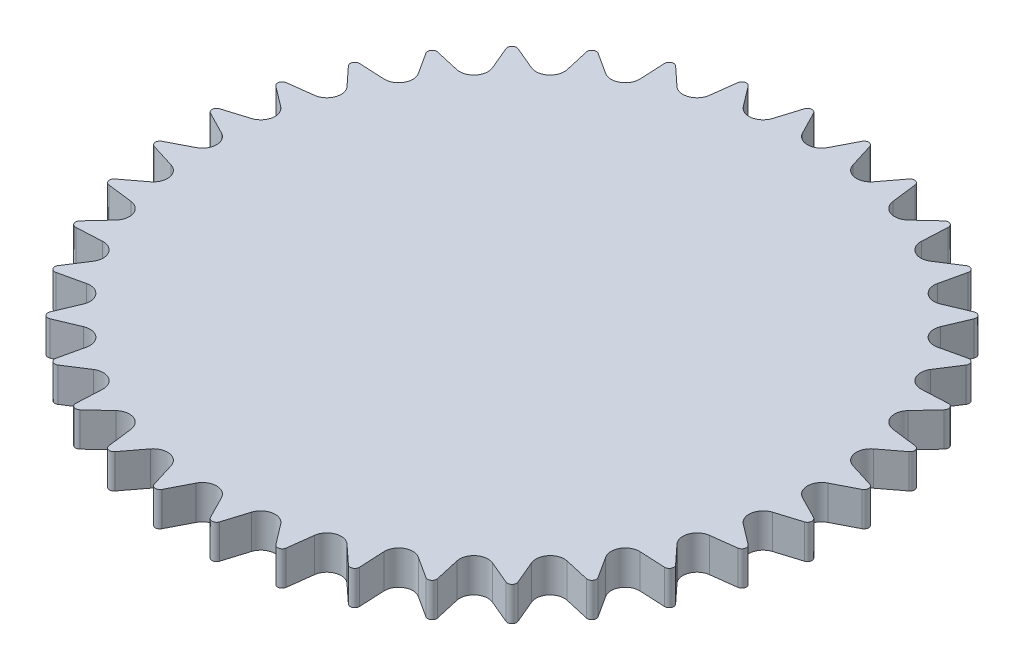
from build123d import *

# Parameters (mm, degrees)
SKETCH_1_R          = 290
BOSS_EXTRUDE1_DEPTH = 30
SKETCH_4_R          = 330.934744746
CUT_EXTRUDE1_DEPTH  = 30


with BuildPart() as part:
    # 草图1 → Boss-Extrude1 (new body)
    with BuildSketch(Plane(origin=(0, 0, 0), x_dir=(1, 0, 0), z_dir=(0, 1, 0))):
        with Locations(Location((0, 0, 0), (0, 0, 270))):
            Circle(SKETCH_1_R)
    extrude(amount=BOSS_EXTRUDE1_DEPTH)

    # 草图4 → Cut-Extrude1 (cut)
    with BuildSketch(Plane(origin=(0, 30, 0), x_dir=(1, 0, 0), z_dir=(0, 1, 0))):
        Circle(SKETCH_4_R)
        with BuildLine():
            Line((-21.368609629, 286.739555153), (-11.118539989, 266.787901567))
            ThreePointArc((-11.118539989, 266.787901567), (0, 260), (11.118539989, 266.787901567))
            Line((11.118539989, 266.787901567), (21.368609629, 286.739555153))
            ThreePointArc((21.368609629, 286.739555153), (22.993156883, 288.413400425), (25.275165397, 288.896462447))
            ThreePointArc((25.275165397, 288.896462447), (27.438622234, 288.024472603), (28.747828783, 286.093957131))
            Line((28.747828783, 286.093957131), (35.377608547, 264.66550808))
            ThreePointArc((35.377608547, 264.66550808), (45.148526193, 256.050015783), (57.276857314, 260.804079666))
            Line((57.276857314, 260.804079666), (70.835773651, 278.672716888))
            ThreePointArc((70.835773651, 278.672716888), (72.726300563, 280.03903302), (75.05752308, 280.118489624))
            ThreePointArc((75.05752308, 280.118489624), (77.036692699, 278.884066928), (77.990778965, 276.755538993))
            Line((77.990778965, 276.755538993), (80.79882635, 254.501387058))
            ThreePointArc((80.79882635, 254.501387058), (88.925237265, 244.320081404), (101.694846313, 246.895857777))
            Line((101.694846313, 246.895857777), (118.150628536, 262.138549136))
            ThreePointArc((118.150628536, 262.138549136), (120.249692402, 263.155821303), (122.559295905, 262.829258241))
            ThreePointArc((122.559295905, 262.829258241), (124.294042239, 261.269910001), (124.864018794, 259.008043847))
            Line((124.864018794, 259.008043847), (123.7650127, 236.604370174))
            ThreePointArc((123.7650127, 236.604370174), (130, 225.166604984), (143.022888867, 225.485830185))
            Line((143.022888867, 225.485830185), (161.875536359, 237.639434218))
            ThreePointArc((161.875536359, 237.639434218), (164.119358186, 238.276753118), (166.337166542, 237.554092844))
            ThreePointArc((166.337166542, 237.554092844), (167.774780201, 235.717199069), (167.943328596, 233.390720353))
            Line((167.943328596, 233.390720353), (162.970661767, 211.51824923))
            ThreePointArc((162.970661767, 211.51824923), (167.124778518, 199.171555211), (180.005253316, 197.224529744))
            Line((180.005253316, 197.224529744), (200.681937923, 205.919765341))
            ThreePointArc((200.681937923, 205.919765341), (203.002340321, 206.157766365), (205.060966544, 205.060966544))
            ThreePointArc((205.060966544, 205.060966544), (206.157766365, 203.002340321), (205.919765341, 200.681937923))
            Line((205.919765341, 200.681937923), (197.224529744, 180.005253316))
            ThreePointArc((197.224529744, 180.005253316), (199.171555211, 167.124778519), (211.51824923, 162.970661767))
            Line((211.51824923, 162.970661767), (233.390720353, 167.943328596))
            ThreePointArc((233.390720353, 167.943328596), (235.717199069, 167.774780201), (237.554092844, 166.337166542))
            ThreePointArc((237.554092844, 166.337166542), (238.276753118, 164.119358186), (237.639434218, 161.875536359))
            Line((237.639434218, 161.875536359), (225.485830185, 143.022888867))
            ThreePointArc((225.485830185, 143.022888867), (225.166604984, 130), (236.604370174, 123.7650127))
            Line((236.604370174, 123.7650127), (259.008043847, 124.864018794))
            ThreePointArc((259.008043847, 124.864018794), (261.269910001, 124.294042239), (262.829258241, 122.559295905))
            ThreePointArc((262.829258241, 122.559295905), (263.155821303, 120.249692402), (262.138549136, 118.150628536))
            Line((262.138549136, 118.150628536), (246.895857777, 101.694846313))
            ThreePointArc((246.895857777, 101.694846313), (244.320081404, 88.925237265), (254.501387058, 80.79882635))
            Line((254.501387058, 80.79882635), (276.755538993, 77.990778965))
            ThreePointArc((276.755538993, 77.990778965), (278.884066928, 77.036692699), (280.118489624, 75.05752308))
            ThreePointArc((280.118489624, 75.05752308), (280.03903302, 72.726300563), (278.672716888, 70.835773651))
            Line((278.672716888, 70.835773651), (260.804079666, 57.276857314))
            ThreePointArc((260.804079666, 57.276857314), (256.050015783, 45.148526193), (264.66550808, 35.377608547))
            Line((264.66550808, 35.377608547), (286.093957131, 28.747828783))
            ThreePointArc((286.093957131, 28.747828783), (288.024472603, 27.438622234), (288.896462447, 25.275165397))
            ThreePointArc((288.896462447, 25.275165397), (288.413400425, 22.993156883), (286.739555153, 21.368609629))
            Line((286.739555153, 21.368609629), (266.787901567, 11.118539989))
            ThreePointArc((266.787901567, 11.118539989), (260, 0), (266.787901567, -11.118539989))
            Line((266.787901567, -11.118539989), (286.739555153, -21.368609629))
            ThreePointArc((286.739555153, -21.368609629), (288.413400425, -22.993156883), (288.896462447, -25.275165397))
            ThreePointArc((288.896462447, -25.275165397), (288.024472603, -27.438622234), (286.093957131, -28.747828783))
            Line((286.093957131, -28.747828783), (264.66550808, -35.377608547))
            ThreePointArc((264.66550808, -35.377608547), (256.050015783, -45.148526193), (260.804079666, -57.276857314))
            Line((260.804079666, -57.276857314), (278.672716888, -70.835773651))
            ThreePointArc((278.672716888, -70.835773651), (280.03903302, -72.726300563), (280.118489624, -75.05752308))
            ThreePointArc((280.118489624, -75.05752308), (278.884066928, -77.036692699), (276.755538993, -77.990778965))
            Line((276.755538993, -77.990778965), (254.501387058, -80.79882635))
            ThreePointArc((254.501387058, -80.79882635), (244.320081404, -88.925237265), (246.895857777, -101.694846313))
            Line((246.895857777, -101.694846313), (262.138549136, -118.150628536))
            ThreePointArc((262.138549136, -118.150628536), (263.155821303, -120.249692402), (262.829258241, -122.559295905))
            ThreePointArc((262.829258241, -122.559295905), (261.269910001, -124.294042239), (259.008043847, -124.864018794))
            Line((259.008043847, -124.864018794), (236.604370174, -123.7650127))
            ThreePointArc((236.604370174, -123.7650127), (225.166604984, -130), (225.485830185, -143.022888867))
            Line((225.485830185, -143.022888867), (237.639434218, -161.875536359))
            ThreePointArc((237.639434218, -161.875536359), (238.276753118, -164.119358186), (237.554092844, -166.337166542))
            ThreePointArc((237.554092844, -166.337166542), (235.717199069, -167.774780201), (233.390720353, -167.943328596))
            Line((233.390720353, -167.943328596), (211.51824923, -162.970661767))
            ThreePointArc((211.51824923, -162.970661767), (199.171555211, -167.124778518), (197.224529744, -180.005253316))
            Line((197.224529744, -180.005253316), (205.919765341, -200.681937923))
            ThreePointArc((205.919765341, -200.681937923), (206.157766365, -203.002340321), (205.060966544, -205.060966544))
            ThreePointArc((205.060966544, -205.060966544), (203.002340321, -206.157766365), (200.681937923, -205.919765341))
            Line((200.681937923, -205.919765341), (180.005253316, -197.224529744))
            ThreePointArc((180.005253316, -197.224529744), (167.124778518, -199.171555211), (162.970661767, -211.51824923))
            Line((162.970661767, -211.51824923), (167.943328596, -233.390720353))
            ThreePointArc((167.943328596, -233.390720353), (167.774780201, -235.717199068), (166.337166542, -237.554092844))
            ThreePointArc((166.337166542, -237.554092844), (164.119358186, -238.276753118), (161.875536359, -237.639434218))
            Line((161.875536359, -237.639434218), (143.022888867, -225.485830185))
            ThreePointArc((143.022888867, -225.485830185), (130, -225.166604984), (123.7650127, -236.604370174))
            Line((123.7650127, -236.604370174), (124.864018794, -259.008043847))
            ThreePointArc((124.864018794, -259.008043847), (124.294042239, -261.269910001), (122.559295905, -262.829258241))
            ThreePointArc((122.559295905, -262.829258241), (120.249692402, -263.155821302), (118.150628536, -262.138549136))
            Line((118.150628536, -262.138549136), (101.694846313, -246.895857777))
            ThreePointArc((101.694846313, -246.895857777), (88.925237265, -244.320081404), (80.79882635, -254.501387058))
            Line((80.79882635, -254.501387058), (77.990778965, -276.755538993))
            ThreePointArc((77.990778965, -276.755538993), (77.036692699, -278.884066928), (75.05752308, -280.118489624))
            ThreePointArc((75.05752308, -280.118489624), (72.726300563, -280.03903302), (70.835773651, -278.672716888))
            Line((70.835773651, -278.672716888), (57.276857314, -260.804079665))
            ThreePointArc((57.276857314, -260.804079665), (45.148526193, -256.050015783), (35.377608547, -264.66550808))
            Line((35.377608547, -264.66550808), (28.747828783, -286.093957131))
            ThreePointArc((28.747828783, -286.093957131), (27.438622234, -288.024472603), (25.275165397, -288.896462447))
            ThreePointArc((25.275165397, -288.896462447), (22.993156883, -288.413400425), (21.368609629, -286.739555153))
            Line((21.368609629, -286.739555153), (11.118539989, -266.787901567))
            ThreePointArc((11.118539989, -266.787901567), (0, -260), (-11.118539989, -266.787901567))
            Line((-11.118539989, -266.787901567), (-21.368609629, -286.739555153))
            ThreePointArc((-21.368609629, -286.739555153), (-22.993156883, -288.413400425), (-25.275165397, -288.896462447))
            ThreePointArc((-25.275165397, -288.896462447), (-27.438622234, -288.024472603), (-28.747828783, -286.093957131))
            Line((-28.747828783, -286.093957131), (-35.377608547, -264.66550808))
            ThreePointArc((-35.377608547, -264.66550808), (-45.148526193, -256.050015783), (-57.276857314, -260.804079665))
            Line((-57.276857314, -260.804079665), (-70.835773651, -278.672716888))
            ThreePointArc((-70.835773651, -278.672716888), (-72.726300563, -280.03903302), (-75.05752308, -280.118489624))
            ThreePointArc((-75.05752308, -280.118489624), (-77.036692699, -278.884066928), (-77.990778965, -276.755538993))
            Line((-77.990778965, -276.755538993), (-80.79882635, -254.501387058))
            ThreePointArc((-80.79882635, -254.501387058), (-88.925237265, -244.320081404), (-101.694846313, -246.895857777))
            Line((-101.694846313, -246.895857777), (-118.150628536, -262.138549136))
            ThreePointArc((-118.150628536, -262.138549136), (-120.249692402, -263.155821302), (-122.559295905, -262.829258241))
            ThreePointArc((-122.559295905, -262.829258241), (-124.294042239, -261.269910001), (-124.864018794, -259.008043847))
            Line((-124.864018794, -259.008043847), (-123.7650127, -236.604370174))
            ThreePointArc((-123.7650127, -236.604370174), (-130, -225.166604984), (-143.022888867, -225.485830185))
            Line((-143.022888867, -225.485830185), (-161.875536359, -237.639434218))
            ThreePointArc((-161.875536359, -237.639434218), (-164.119358186, -238.276753118), (-166.337166542, -237.554092844))
            ThreePointArc((-166.337166542, -237.554092844), (-167.774780201, -235.717199068), (-167.943328596, -233.390720353))
            Line((-167.943328596, -233.390720353), (-162.970661767, -211.51824923))
            ThreePointArc((-162.970661767, -211.51824923), (-167.124778518, -199.171555211), (-180.005253316, -197.224529744))
            Line((-180.005253316, -197.224529744), (-200.681937923, -205.919765341))
            ThreePointArc((-200.681937923, -205.919765341), (-203.002340321, -206.157766365), (-205.060966544, -205.060966544))
            ThreePointArc((-205.060966544, -205.060966544), (-206.157766365, -203.002340321), (-205.919765341, -200.681937923))
            Line((-205.919765341, -200.681937923), (-197.224529744, -180.005253316))
            ThreePointArc((-197.224529744, -180.005253316), (-199.171555211, -167.124778518), (-211.51824923, -162.970661767))
            Line((-211.51824923, -162.970661767), (-233.390720353, -167.943328596))
            ThreePointArc((-233.390720353, -167.943328596), (-235.717199069, -167.774780201), (-237.554092844, -166.337166542))
            ThreePointArc((-237.554092844, -166.337166542), (-238.276753118, -164.119358186), (-237.639434218, -161.875536359))
            Line((-237.639434218, -161.875536359), (-225.485830185, -143.022888867))
            ThreePointArc((-225.485830185, -143.022888867), (-225.166604984, -130), (-236.604370174, -123.7650127))
            Line((-236.604370174, -123.7650127), (-259.008043847, -124.864018794))
            ThreePointArc((-259.008043847, -124.864018794), (-261.269910001, -124.294042239), (-262.829258241, -122.559295905))
            ThreePointArc((-262.829258241, -122.559295905), (-263.155821303, -120.249692402), (-262.138549136, -118.150628536))
            Line((-262.138549136, -118.150628536), (-246.895857777, -101.694846313))
            ThreePointArc((-246.895857777, -101.694846313), (-244.320081404, -88.925237265), (-254.501387058, -80.79882635))
            Line((-254.501387058, -80.79882635), (-276.755538993, -77.990778965))
            ThreePointArc((-276.755538993, -77.990778965), (-278.884066928, -77.036692699), (-280.118489624, -75.05752308))
            ThreePointArc((-280.118489624, -75.05752308), (-280.03903302, -72.726300563), (-278.672716888, -70.835773651))
            Line((-278.672716888, -70.835773651), (-260.804079666, -57.276857314))
            ThreePointArc((-260.804079666, -57.276857314), (-256.050015783, -45.148526193), (-264.66550808, -35.377608547))
            Line((-264.66550808, -35.377608547), (-286.093957131, -28.747828783))
            ThreePointArc((-286.093957131, -28.747828783), (-288.024472603, -27.438622234), (-288.896462447, -25.275165397))
            ThreePointArc((-288.896462447, -25.275165397), (-288.413400425, -22.993156883), (-286.739555153, -21.368609629))
            Line((-286.739555153, -21.368609629), (-266.787901567, -11.118539989))
            ThreePointArc((-266.787901567, -11.118539989), (-260, 0), (-266.787901567, 11.118539989))
            Line((-266.787901567, 11.118539989), (-286.739555153, 21.368609629))
            ThreePointArc((-286.739555153, 21.368609629), (-288.413400425, 22.993156883), (-288.896462447, 25.275165397))
            ThreePointArc((-288.896462447, 25.275165397), (-288.024472603, 27.438622234), (-286.093957131, 28.747828783))
            Line((-286.093957131, 28.747828783), (-264.66550808, 35.377608547))
            ThreePointArc((-264.66550808, 35.377608547), (-256.050015783, 45.148526193), (-260.804079666, 57.276857314))
            Line((-260.804079666, 57.276857314), (-278.672716888, 70.835773651))
            ThreePointArc((-278.672716888, 70.835773651), (-280.03903302, 72.726300563), (-280.118489624, 75.05752308))
            ThreePointArc((-280.118489624, 75.05752308), (-278.884066928, 77.036692699), (-276.755538993, 77.990778965))
            Line((-276.755538993, 77.990778965), (-254.501387058, 80.79882635))
            ThreePointArc((-254.501387058, 80.79882635), (-244.320081404, 88.925237265), (-246.895857777, 101.694846313))
            Line((-246.895857777, 101.694846313), (-262.138549136, 118.150628536))
            ThreePointArc((-262.138549136, 118.150628536), (-263.155821303, 120.249692402), (-262.829258241, 122.559295905))
            ThreePointArc((-262.829258241, 122.559295905), (-261.269910001, 124.294042239), (-259.008043847, 124.864018794))
            Line((-259.008043847, 124.864018794), (-236.604370174, 123.7650127))
            ThreePointArc((-236.604370174, 123.7650127), (-225.166604984, 130), (-225.485830185, 143.022888867))
            Line((-225.485830185, 143.022888867), (-237.639434218, 161.875536359))
            ThreePointArc((-237.639434218, 161.875536359), (-238.276753118, 164.119358186), (-237.554092844, 166.337166542))
            ThreePointArc((-237.554092844, 166.337166542), (-235.717199069, 167.774780201), (-233.390720353, 167.943328596))
            Line((-233.390720353, 167.943328596), (-211.51824923, 162.970661767))
            ThreePointArc((-211.51824923, 162.970661767), (-199.171555211, 167.124778519), (-197.224529744, 180.005253316))
            Line((-197.224529744, 180.005253316), (-205.919765341, 200.681937923))
            ThreePointArc((-205.919765341, 200.681937923), (-206.157766365, 203.002340321), (-205.060966544, 205.060966544))
            ThreePointArc((-205.060966544, 205.060966544), (-203.002340321, 206.157766365), (-200.681937923, 205.919765341))
            Line((-200.681937923, 205.919765341), (-180.005253316, 197.224529744))
            ThreePointArc((-180.005253316, 197.224529744), (-167.124778518, 199.171555211), (-162.970661767, 211.51824923))
            Line((-162.970661767, 211.51824923), (-167.943328596, 233.390720353))
            ThreePointArc((-167.943328596, 233.390720353), (-167.774780201, 235.717199069), (-166.337166542, 237.554092844))
            ThreePointArc((-166.337166542, 237.554092844), (-164.119358186, 238.276753118), (-161.875536359, 237.639434218))
            Line((-161.875536359, 237.639434218), (-143.022888867, 225.485830185))
            ThreePointArc((-143.022888867, 225.485830185), (-130, 225.166604984), (-123.7650127, 236.604370174))
            Line((-123.7650127, 236.604370174), (-124.864018794, 259.008043847))
            ThreePointArc((-124.864018794, 259.008043847), (-124.294042239, 261.269910001), (-122.559295905, 262.829258241))
            ThreePointArc((-122.559295905, 262.829258241), (-120.249692402, 263.155821303), (-118.150628536, 262.138549136))
            Line((-118.150628536, 262.138549136), (-101.694846313, 246.895857777))
            ThreePointArc((-101.694846313, 246.895857777), (-88.925237265, 244.320081404), (-80.79882635, 254.501387058))
            Line((-80.79882635, 254.501387058), (-77.990778965, 276.755538993))
            ThreePointArc((-77.990778965, 276.755538993), (-77.036692699, 278.884066928), (-75.05752308, 280.118489624))
            ThreePointArc((-75.05752308, 280.118489624), (-72.726300563, 280.03903302), (-70.835773651, 278.672716888))
            Line((-70.835773651, 278.672716888), (-57.276857314, 260.804079666))
            ThreePointArc((-57.276857314, 260.804079666), (-45.148526193, 256.050015783), (-35.377608547, 264.66550808))
            Line((-35.377608547, 264.66550808), (-28.747828783, 286.093957131))
            ThreePointArc((-28.747828783, 286.093957131), (-27.438622234, 288.024472603), (-25.275165397, 288.896462447))
            ThreePointArc((-25.275165397, 288.896462447), (-22.993156883, 288.413400425), (-21.368609629, 286.739555153))
        make_face(mode=Mode.SUBTRACT)
    extrude(amount=-CUT_EXTRUDE1_DEPTH, mode=Mode.SUBTRACT)


solid = part.part
